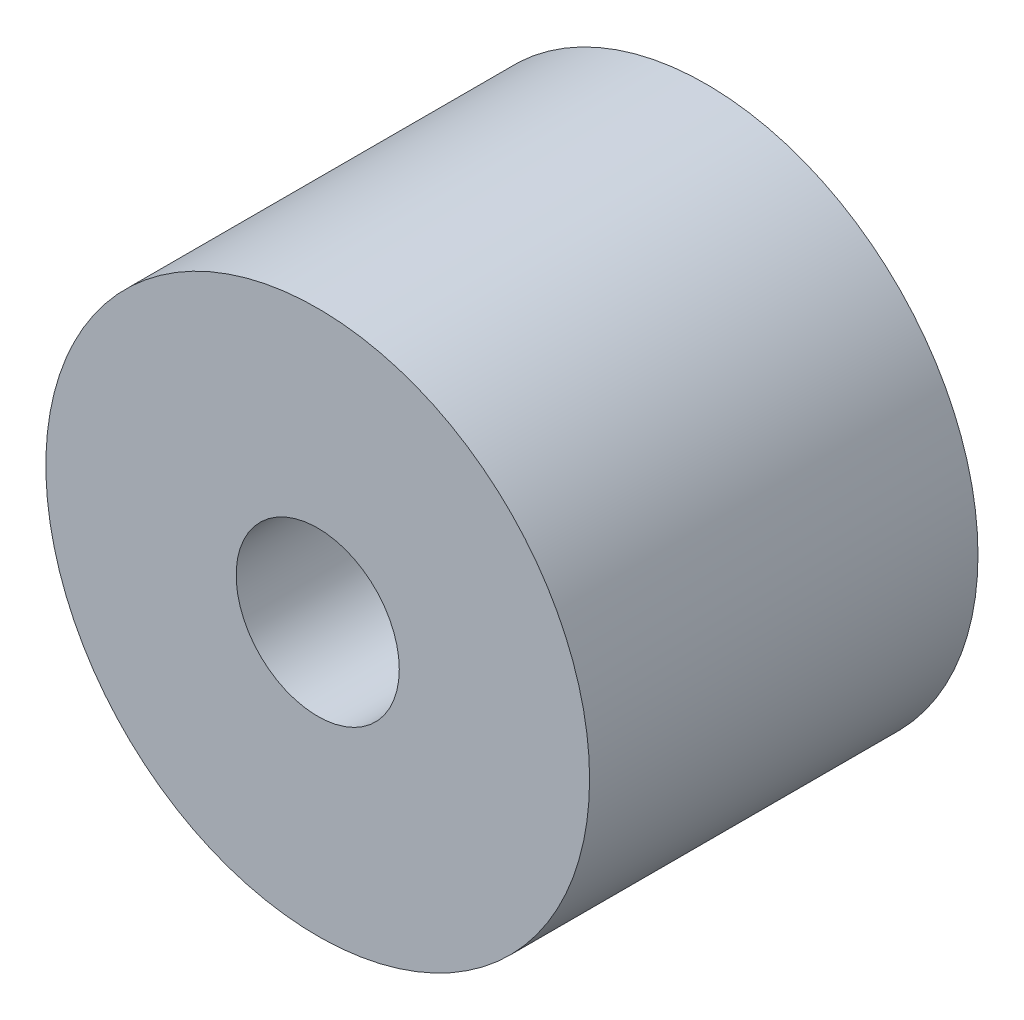
from build123d import *

# Parameters (mm, degrees)
SKETCH_1_R         = 7
EXTRUDE_1_DEPTH    = 10
HOLE_WIZARD_M5_1_D = 4.2


with BuildPart() as part:
    # 草图1 → 凸台-拉伸1 (new body)
    with BuildSketch(Plane.XY):
        Circle(SKETCH_1_R)
    extrude(amount=EXTRUDE_1_DEPTH)

    # M5 螺纹孔1 (through all)
    with Locations(Plane.XY.offset(10)):
        with Locations((0, 0)):
            Hole(HOLE_WIZARD_M5_1_D / 2)


solid = part.part
